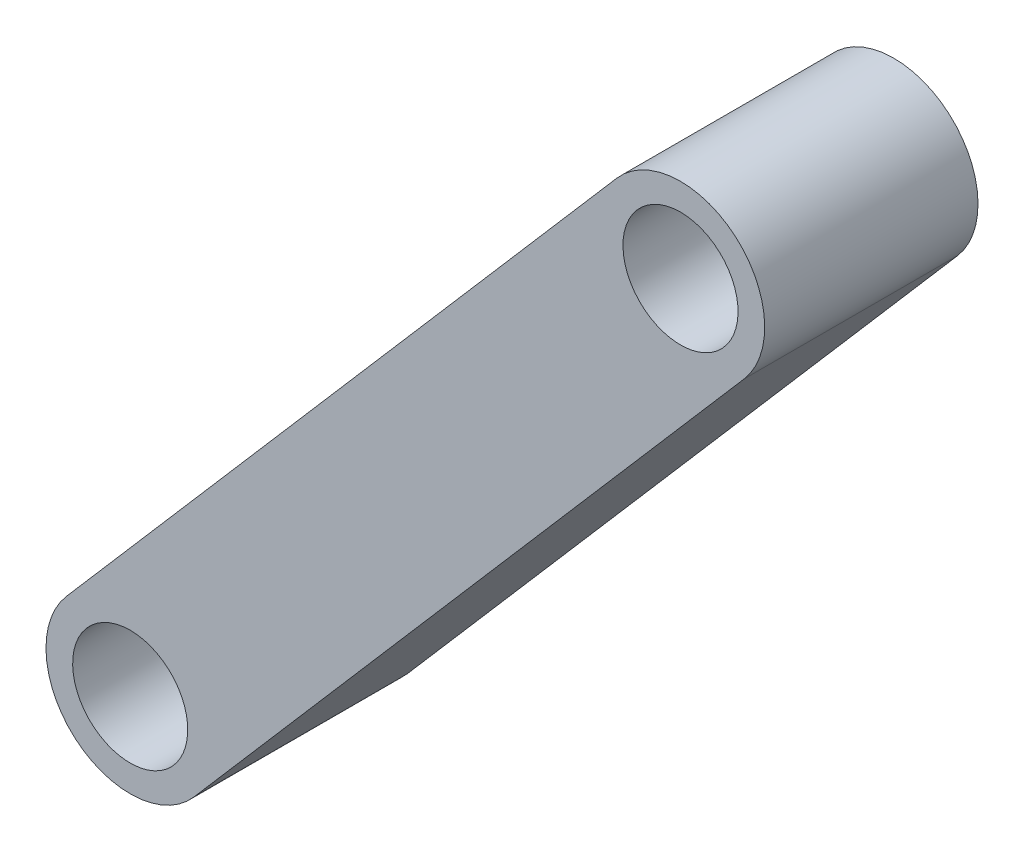
SolidWorks part; units mm, degrees
ref_plane "Front Plane" through (0, 0, 0) normal (0, 0, 1) x (1, 0, 0)
ref_plane "Top Plane" through (0, 0, 0) normal (0, 1, 0) x (1, 0, 0)
ref_plane "Right Plane" through (0, 0, 0) normal (1, 0, 0) x (0, 0, -1)
sketch "Sketch1" plane through (0, 0, 0) normal (0, 0, 1) x (1, 0, 0)
  line L0 (15.24, -3.25) -> (40.1417, 25.586) construction
  line L1 (12.3564, -0.7598) -> (37.258, 28.0762)
  line L2 (18.1236, -5.7402) -> (43.0253, 23.0959)
  line L8 (19.05, 3.5) -> (10.16, 3.5)
  line L9 (10.16, 3.5) -> (10.16, -10)
  line L10 (10.16, -10) -> (19.05, -10)
  line L11 (19.05, -10) -> (19.05, 3.5)
  circle A2 centre (15.24, -3.25) radius 2.6035
  circle A3 centre (40.1417, 25.586) radius 2.6035
  arc A4 (12.3564, -0.7598) -> (18.1236, -5.7402) centre (15.24, -3.25) ccw
  arc A5 (43.0253, 23.0959) -> (37.258, 28.0762) centre (40.1417, 25.586) ccw
  point P10 (27.6908, 11.168)
  dimension "D3" = 5.207
  dimension "D4" = 5.207
  dimension "D2" = 7.62
  dimension "D1" = 38.1
extrude "Boss-Extrude1" add sketch "Sketch1" along normal up to surface (9.652 mm away)
